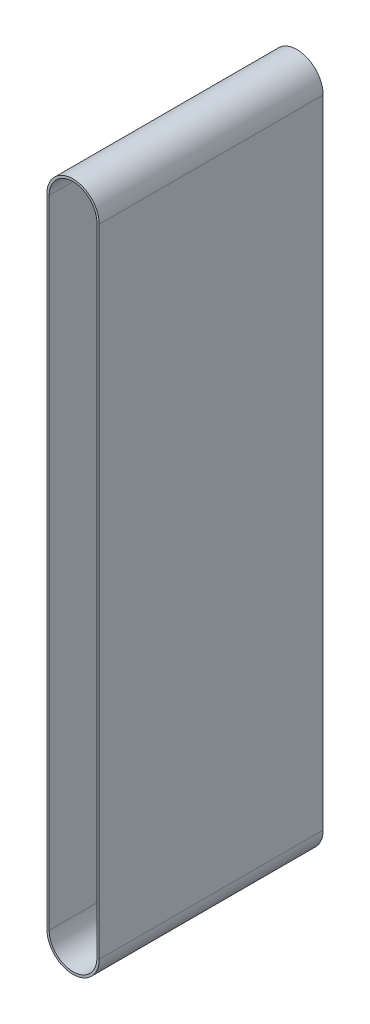
SolidWorks part; units mm, degrees
ref_plane "前视基准面" through (0, 0, 0) normal (0, 0, 1) x (1, 0, 0)
ref_plane "上视基准面" through (0, 0, 0) normal (0, 1, 0) x (1, 0, 0)
ref_plane "右视基准面" through (0, 0, 0) normal (1, 0, 0) x (0, 0, -1)
sketch "草图2" plane through (0, 0, 0) normal (0, 0, 1) x (1, 0, 0)
  line L0 (0, 0) -> (1, 0) construction
  line L1 (0, 0) -> (0, 1) construction
  line L2 (-20.25, 0) -> (-20.25, 540)
  line L3 (20.25, 540) -> (20.25, 0)
  arc A0 (20.25, 0) -> (-20.25, 0) centre (0, 0) cw
  arc A1 (-20.25, 540) -> (20.25, 540) centre (0, 540) cw
extrude "拉伸-薄壁1" add sketch "草图2" along normal mid plane 190 thin thin type one direction wall 2
